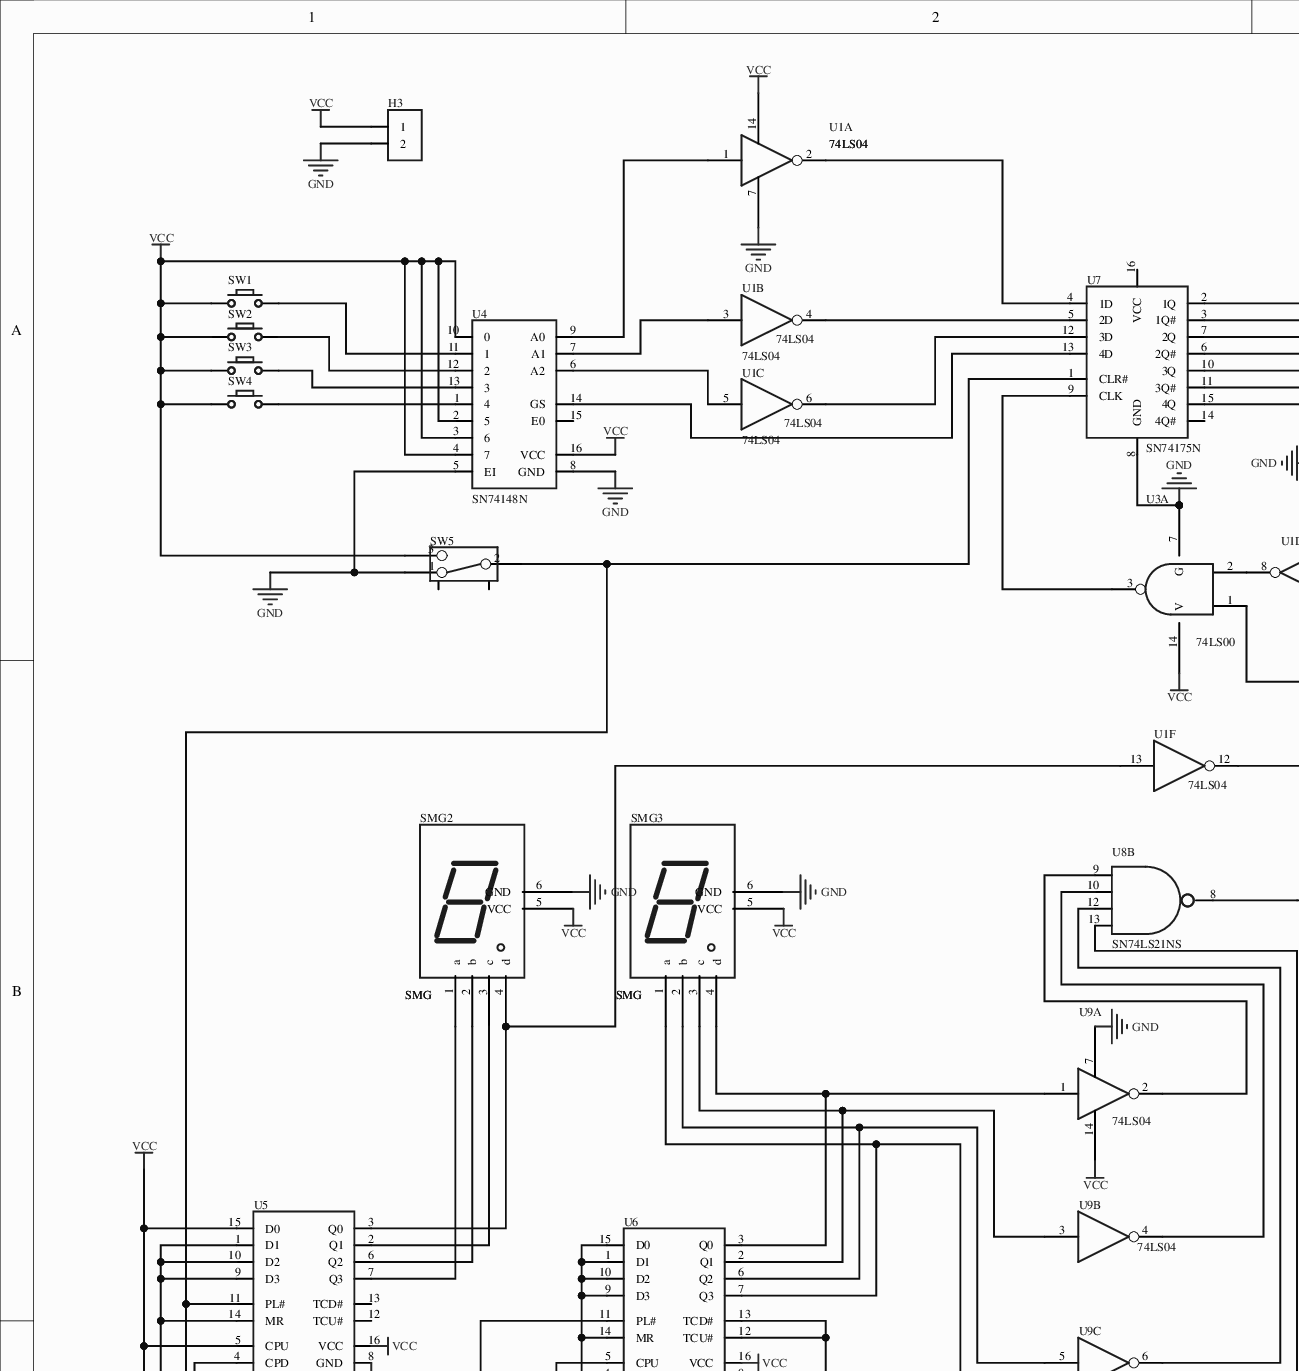
[diagram p0: MISC52149-3.schdoc, top left]
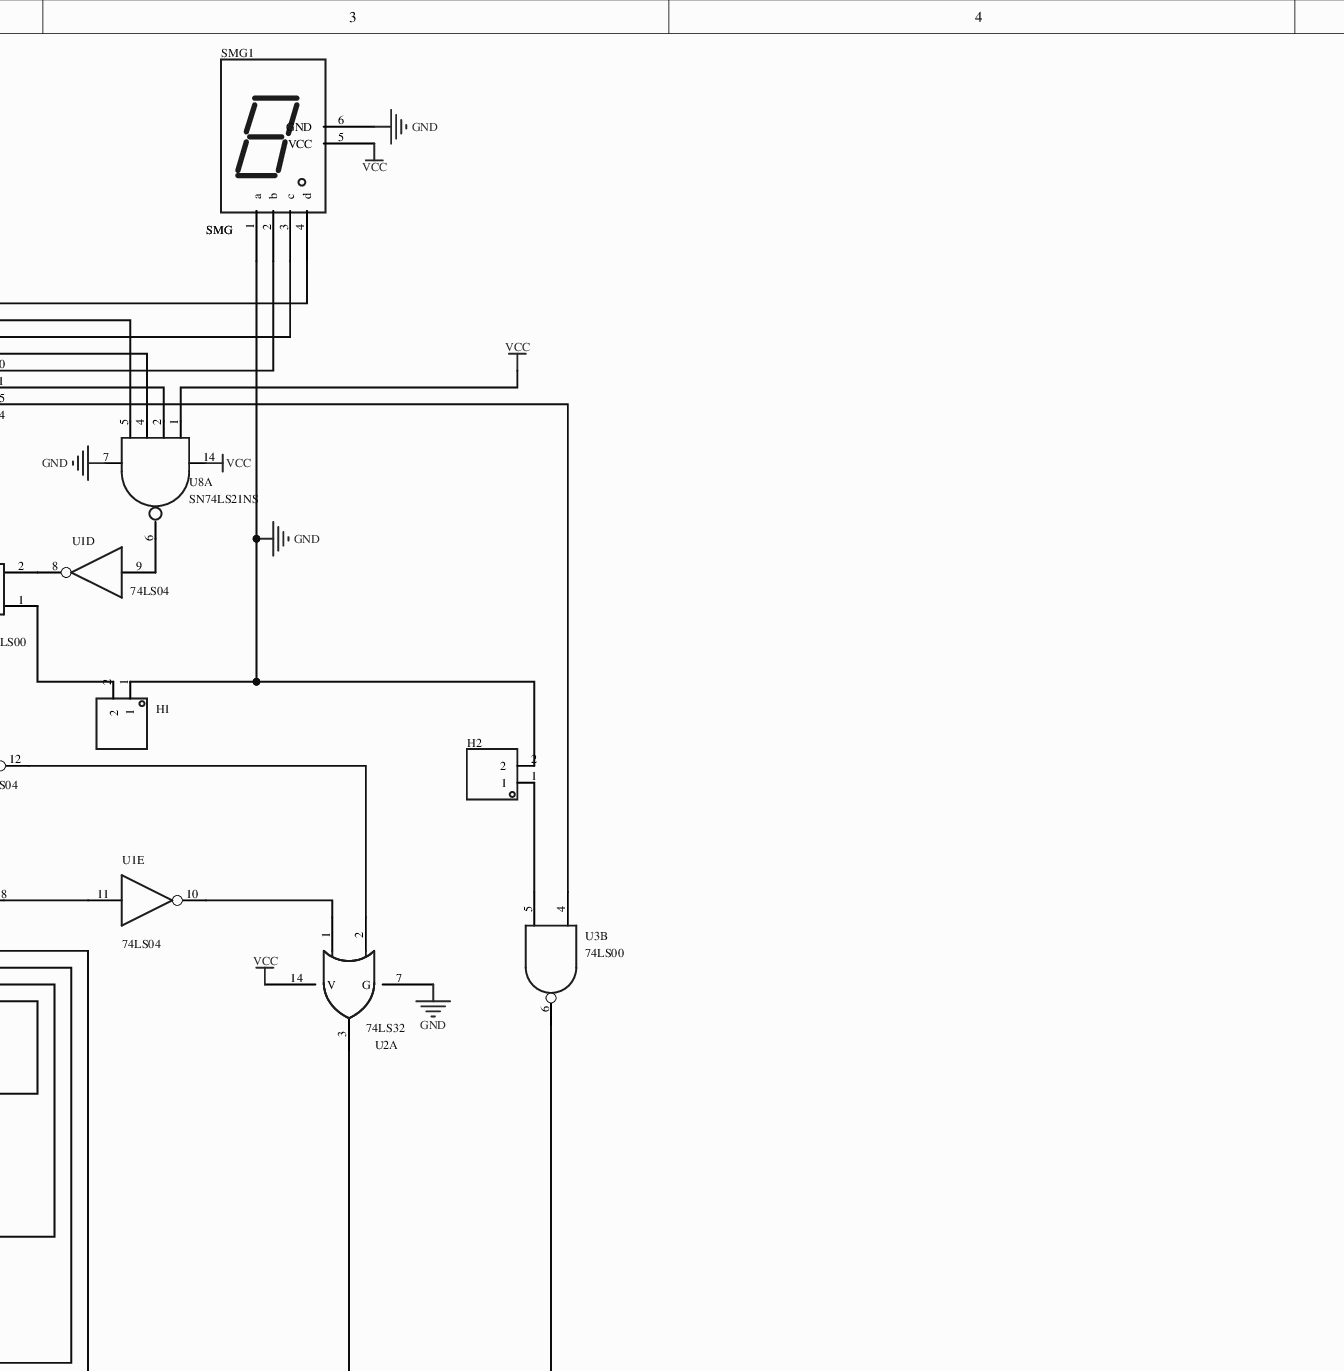
[diagram p1: MISC52149-3.schdoc, top middle]
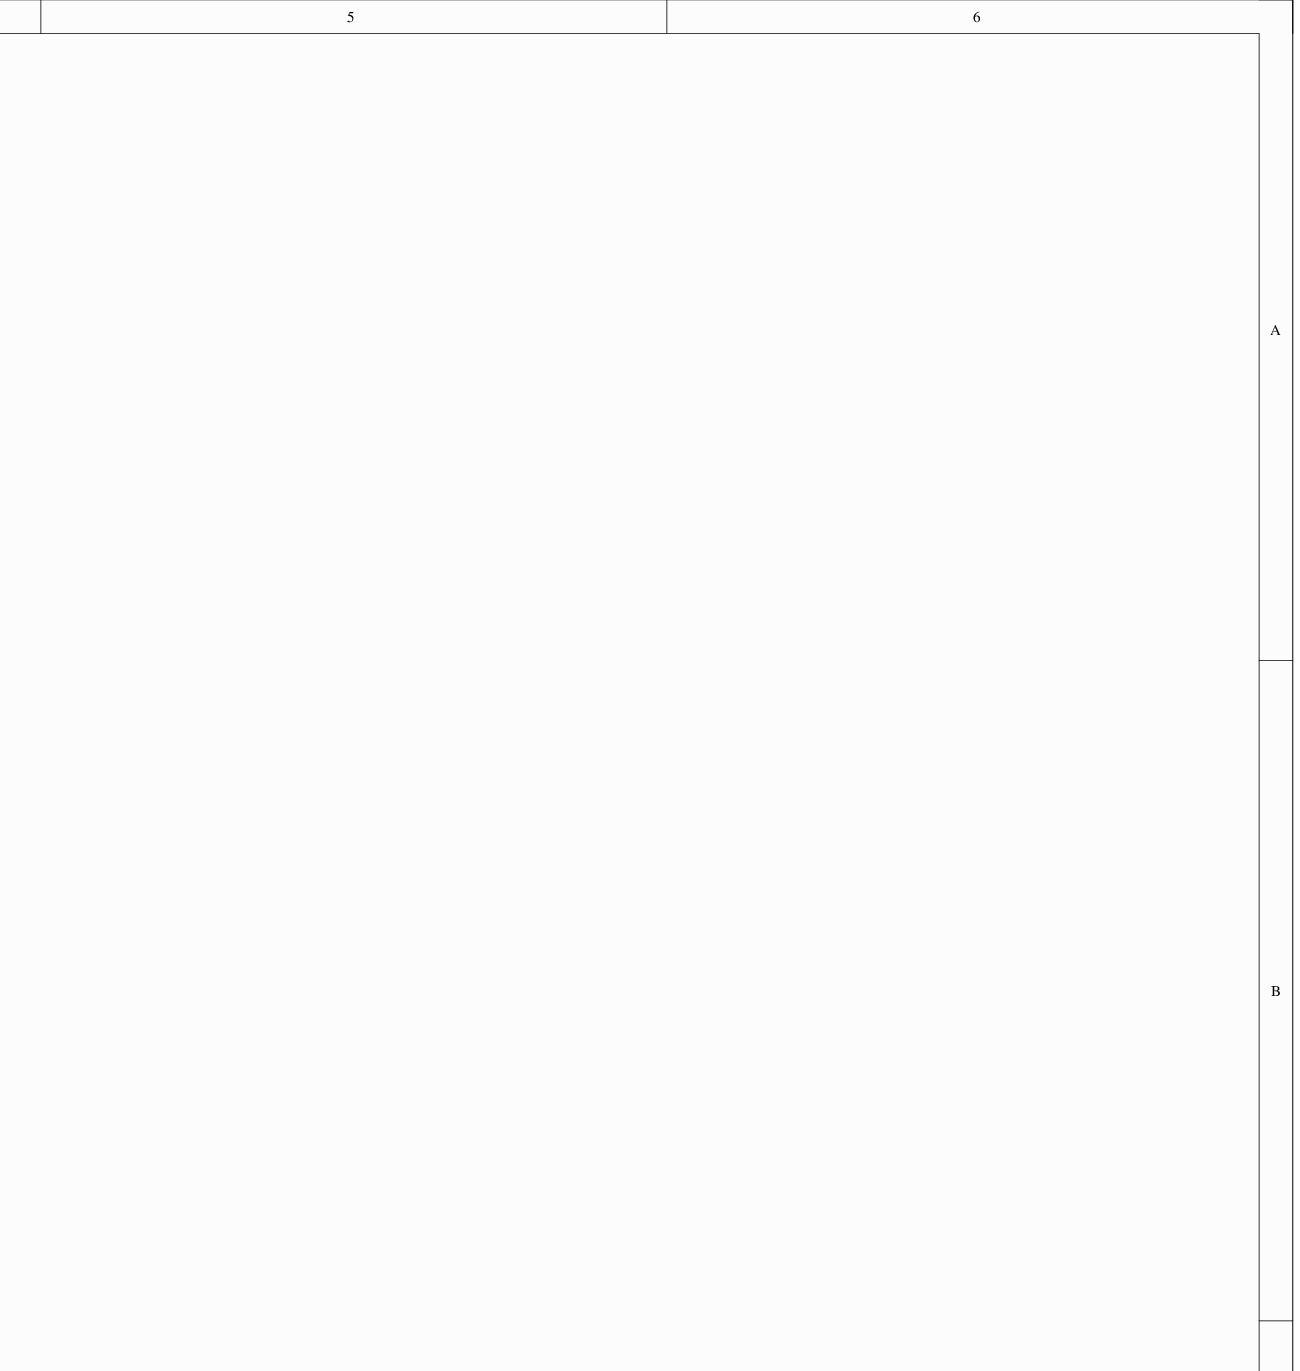
[diagram p2: MISC52149-3.schdoc, top right]
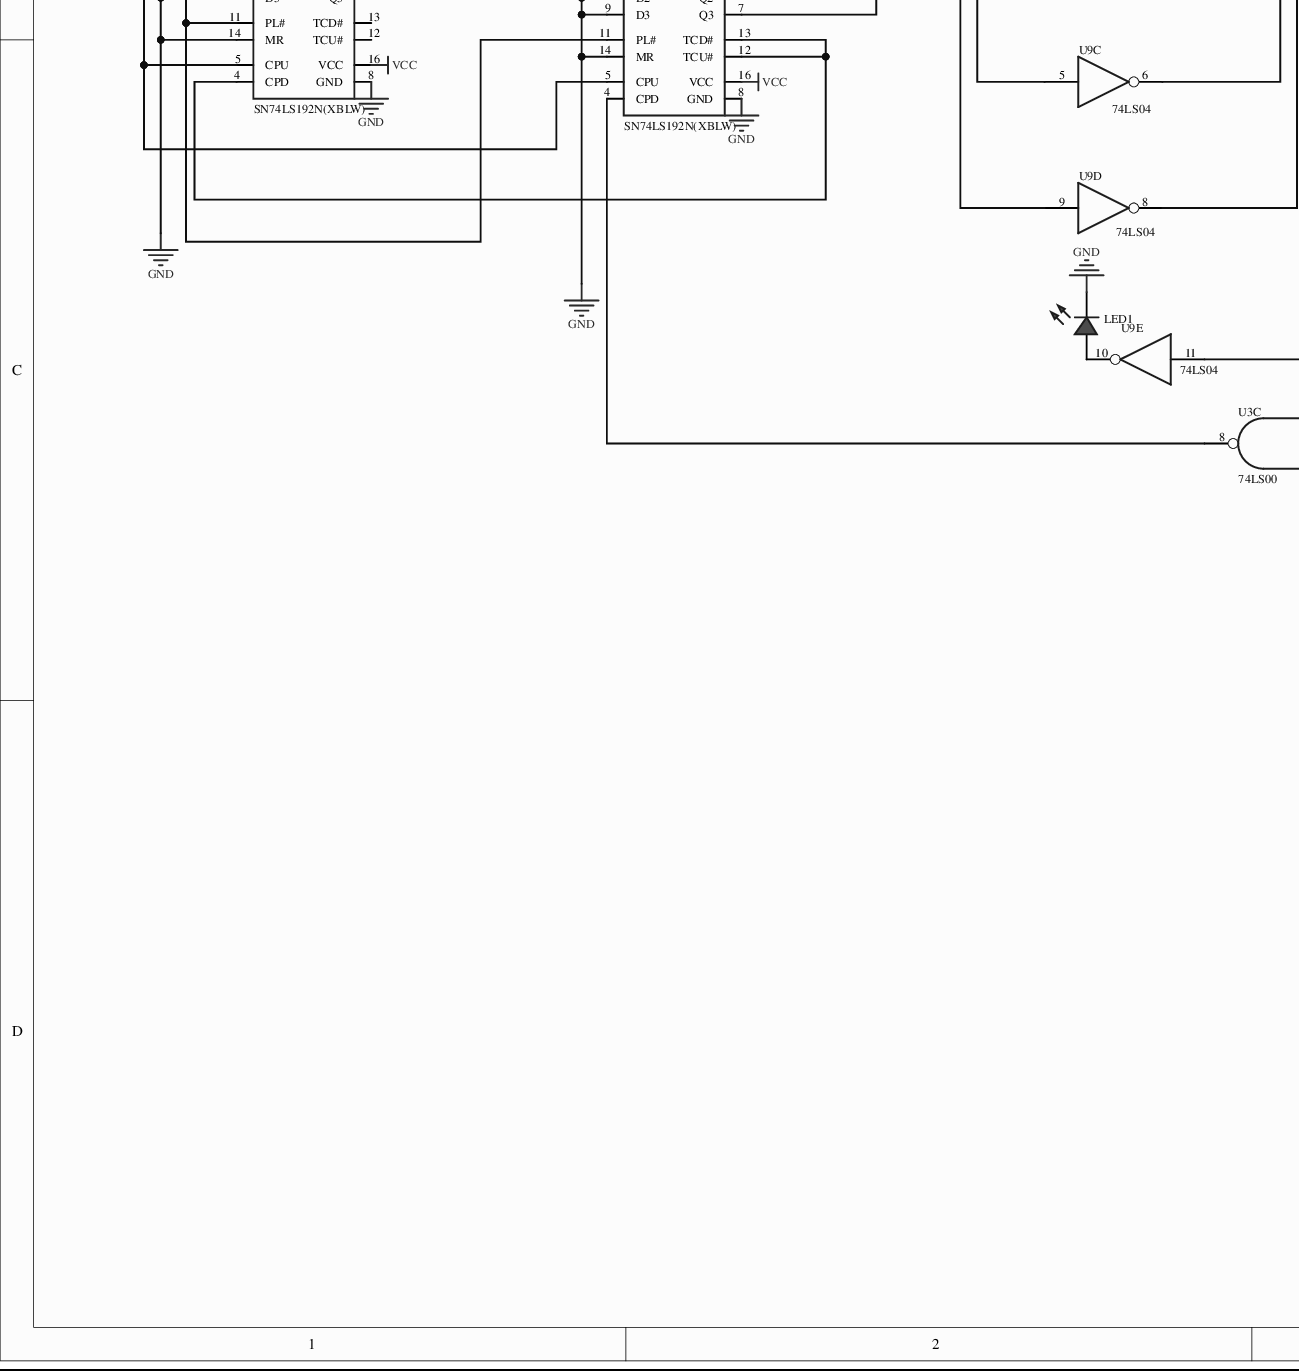
[diagram p3: MISC52149-3.schdoc, bottom left]
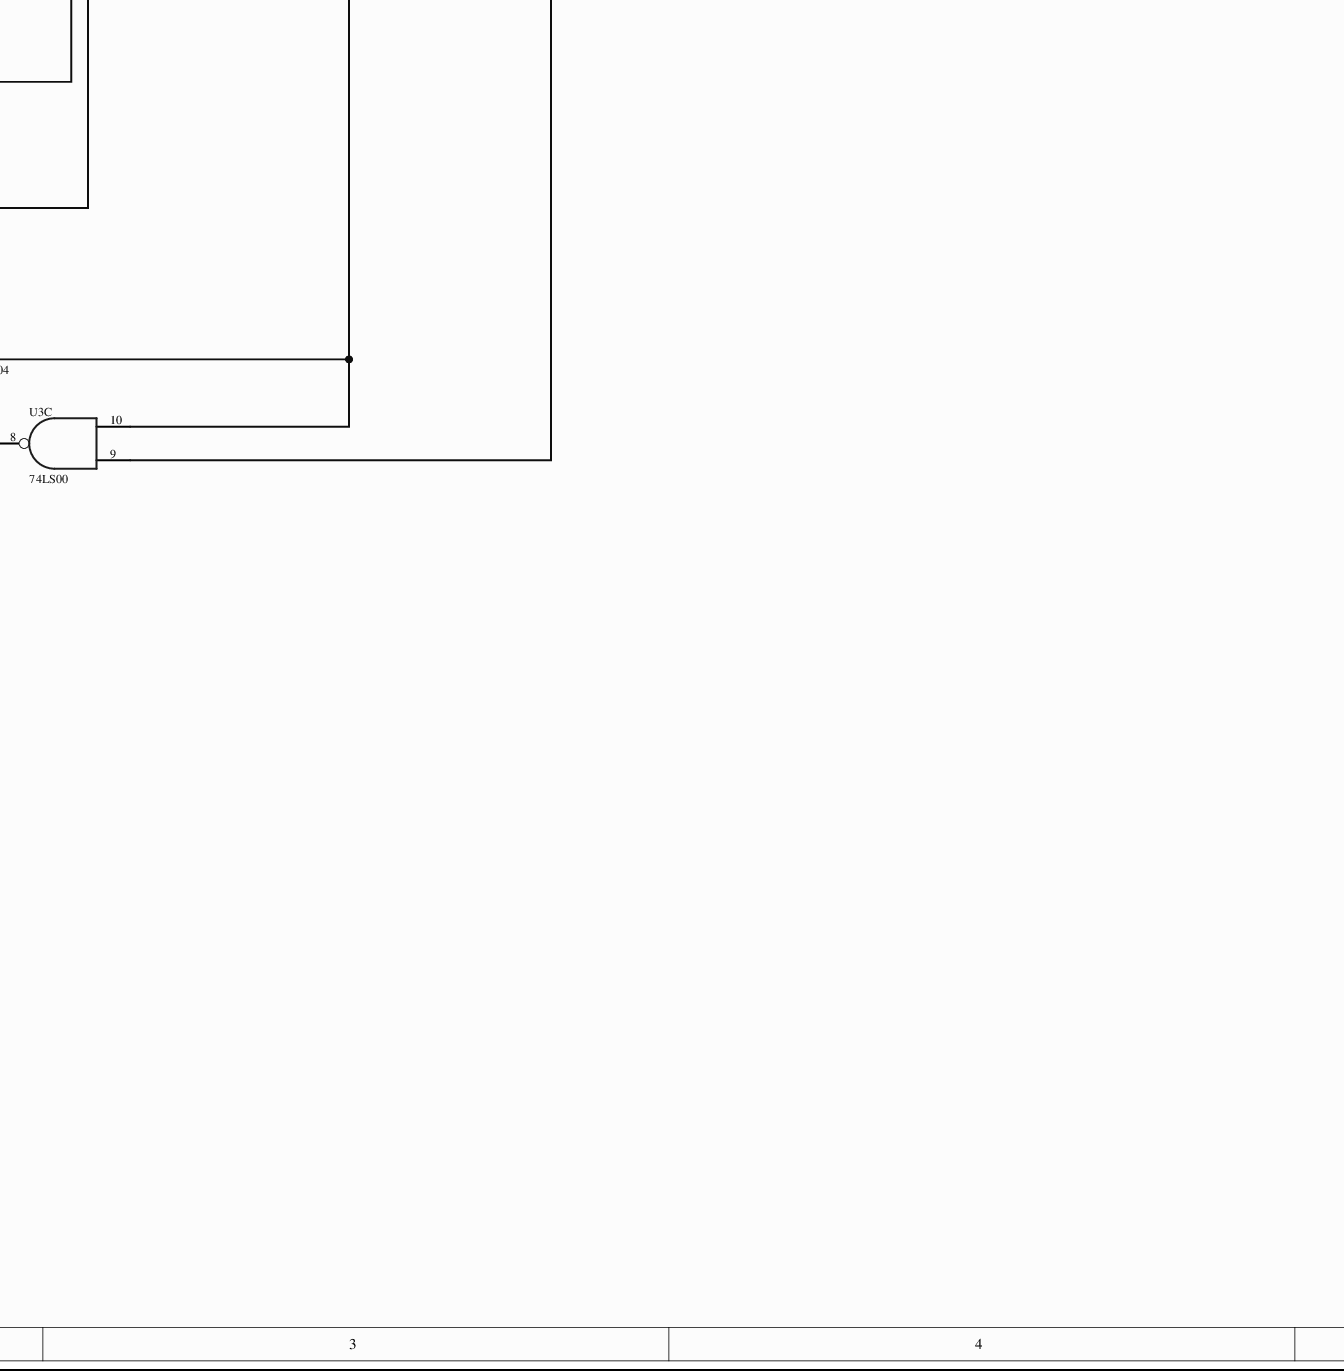
[diagram p4: MISC52149-3.schdoc, bottom middle]
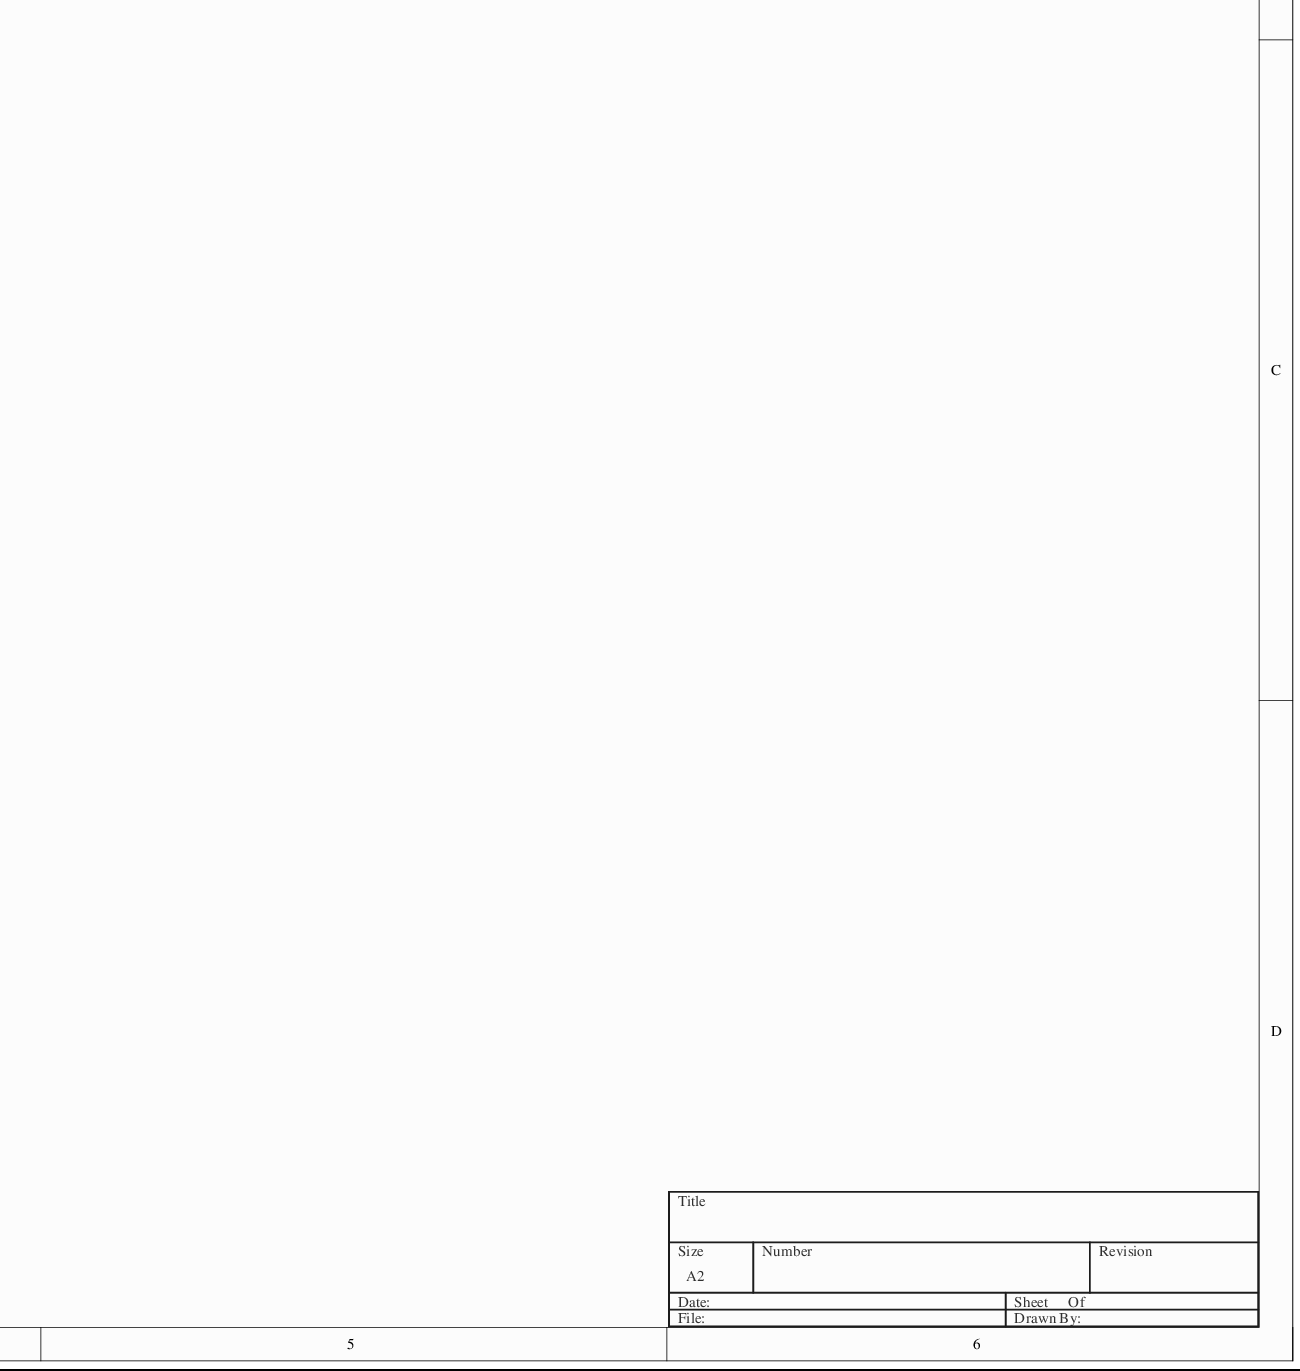
[diagram p5: MISC52149-3.schdoc, bottom right]
# Altium project MISC52149-2.PrjPcb
1 sheet, 21 parts. Net scope: global (net labels, ports and power ports of the same name join across sheets).
Board file: MISC52149.pcbdoc

## Sheet MISC52149-3.schdoc
size 566 x 399 mm

### Parts
H1  (no value)  [HDR-TH_2P-P2.54-V-M-1]
H2  (no value)  [HDR-TH_2P-P2.54-V-M-1]
H3  (no value)  [HDR-TH_2P-P2.54-V-F]
LED1  (no value)  [LED_TH-3mm]
SMG1  SMG  [B含CD译码器的数码管]
SMG2  SMG  [B含CD译码器的数码管]
SMG3  SMG  [B含CD译码器的数码管]
SW1  (no value)  [Key_TH_3.5x6x4.3]
SW2  (no value)  [Key_TH_3.5x6x4.3]
SW3  (no value)  [Key_TH_3.5x6x4.3]
SW4  (no value)  [Key_TH_3.5x6x4.3]
SW5  (no value)  [拨动开关]
U1  74LS04  [DIP-014]  (parts A,B,C,D,E,F of 6)
U2  74LS32  [DIP-014]  (part A of 4)
U3  74LS00  [DIP-014]  (parts A,B,C of 4)
U4  SN74148N  [PDIP-16_L19.3-W6.4-P2.54-LS7.9-BL]
U5  SN74LS192N(XBLW)  [PDIP-16_L19.3-W6.4-P2.54-LS7.94-BL]
U6  SN74LS192N(XBLW)  [PDIP-16_L19.3-W6.4-P2.54-LS7.94-BL]
U7  SN74175N  [DIP-16_L19.3-W6.4-P2.54-LS7.6-BL]
U8  SN74LS21NS  [SOIC-14_L10.0-W5.5-P1.27-LS7.8-BL]  (parts A,B of 2)
U9  74LS04  [DIP-014]  (parts A,B,C,D,E of 6)

### Nets
GND: H1.1 H2.2 H3.2 LED1.2(A) SMG1.1(a) SMG1.6(GND) SMG2.6(GND) SMG3.6(GND) SW5.1 U1.7 U2.7(G) U3.7(G) U4.5(EI) U4.8(GND) U5.1(D1) U5.8(GND) U5.9(D3) U5.10(D2) U5.14(MR) U6.1(D1) U6.8(GND) U6.9(D3) U6.10(D2) U6.14(MR) U6.15(D0) U7.8(GND) U8.7(GND) U9.7
VCC: H3.1 SMG1.5(VCC) SMG2.5(VCC) SMG3.5(VCC) SW1.A SW2.A SW3.A SW4.A SW5.3 U1.14 U2.14(V) U3.14(V) U4.2(5) U4.3(6) U4.4(7) U4.10(0) U4.16(VCC) U5.5(CPU) U5.15(D0) U5.16(VCC) U6.5(CPU) U6.16(VCC) U8.1(1A) U8.14(VCC) U9.14
NetH1_2: H1.2 U3.1(A)
NetH2_1: H2.1 U3.5(B)
NetLED1_1: LED1.1(C) U9.10(Y)
NetSMG1_2: SMG1.2(b) U7.10(3Q)
NetSMG1_3: SMG1.3(c) U7.7(2Q)
NetSMG1_4: SMG1.4(d) U7.2(1Q)
NetSMG2_1: SMG2.1(a) U5.7(Q3)
NetSMG2_2: SMG2.2(b) U5.6(Q2)
NetSMG2_3: SMG2.3(c) U5.2(Q1)
NetSMG2_4: SMG2.4(d) U1.13(A) U5.3(Q0)
NetSMG3_1: SMG3.1(a) U6.7(Q3) U9.9(A)
NetSMG3_2: SMG3.2(b) U6.6(Q2) U9.5(A)
NetSMG3_3: SMG3.3(c) U6.2(Q1) U9.3(A)
NetSMG3_4: SMG3.4(d) U6.3(Q0) U9.1(A)
NetSW1_B: SW1.B U4.11(1)
NetSW2_B: SW2.B U4.12(2)
NetSW3_B: SW3.B U4.13(3)
NetSW4_B: SW4.B U4.1(4)
NetSW5_2: SW5.2 U5.11(PL#) U6.11(PL#) U7.1(CLR#)
NetU1_1: U1.1(A) U4.9(A0)
NetU1_2: U1.2(Y) U7.4(1D)
NetU1_3: U1.3(A) U4.7(A1)
NetU1_4: U1.4(Y) U7.5(2D)
NetU1_5: U1.5(A) U4.6(A2)
NetU1_6: U1.6(Y) U7.12(3D)
NetU1_8: U1.8(Y) U3.2(B)
NetU1_9: U1.9(A) U8.6(1Y)
NetU1_10: U1.10(Y) U2.1(A)
NetU1_11: U1.11(A) U8.8(2Y)
NetU1_12: U1.12(Y) U2.2(B)
NetU2_3: U2.3(Y) U3.10(B) U9.11(A)
NetU3_3: U3.3(Y) U7.9(CLK)
NetU3_4: U3.4(A) U7.15(4Q)
NetU3_6: U3.6(Y) U3.9(A)
NetU3_8: U3.8(Y) U6.4(CPD)
NetU4_14: U4.14(GS) U7.13(4D)
NetU5_4: U5.4(CPD) U6.12(TCU#) U6.13(TCD#)
NetU7_3: U7.3(1Q#) U8.5(1D)
NetU7_6: U7.6(2Q#) U8.4(1C)
NetU7_11: U7.11(3Q#) U8.2(1B)
NetU8_9: U8.9(2A) U9.2(Y)
NetU8_10: U8.10(2B) U9.4(Y)
NetU8_12: U8.12(2C) U9.6(Y)
NetU8_13: U8.13(2D) U9.8(Y)

Not connected (* = marked no-connect by the designer): SW5 4 5; U4 15(E0)*; U5 12(TCU#)* 13(TCD#)*; U7 14(4Q#) 16(VCC)

### Notes on the sheet
- Title
- File:
- Date:
- Size
- A2
- Number
- Drawn By:
- Sheet
- Of
- Revision

### Library data of the parts
H1 H2 = HDR-M_2.54_1x2P: Symbol: 210S-1*2P L=11.6MMGold-plated black; ConvertToPcb: yes; ModelId: 79b2e9f2d70a4d68a1b7098f27c6d4c50819f05c4eef4c71ace90d822a990e87; ModelName: HDR-M-2.54_1x2; ModelTransform: 200,100,0,0,0,0,0,0,-118.11; Device: HDR-M_2.54_1x2P; AddInBom: yes; SupplierPart: C124375; Supplier Footprint: 插件; FootprintName: HDR-TH_2P-P2.54-V-M-1
H3 = HDR-F_2.54_1x2P: Symbol: Header-Female-2.54_1x2; ConvertToPcb: yes; ModelId: a9450ef445564560a104363b9aacde4e0819f05c4eef4c71ace90d822a990e87; ModelName: HDR-TH_2P-P2.54-F-LI-1X2P; ModelTransform: 215.7476,98.425,0,0,0,0,0,0,-129.921; Device: HDR-F_2.54_1x2P; AddInBom: yes; SupplierPart: C49661; Supplier Footprint: 插件; FootprintName: HDR-TH_2P-P2.54-V-F
LED1 = LED_TH-R_3mm: ConvertToPcb: yes; ModelId: a497c992633541038a38947cdc58012f0819f05c4eef4c71ace90d822a990e87; ModelName: LED-TH-3mm_R; ModelTransform: 141.274,153.327,0,0,0,0,-5.984,0,-137.795; Symbol: LED_TH-R; Device: LED_TH-R_3mm; AddInBom: yes; FootprintName: LED_TH-3mm; Supplier Footprint: 插件
SMG1-SMG3 = SMG: Origin Footprint: BCD-decoder display; AddInBom: yes; Symbol: SMG; Device: SMG; Design Item ID: SMG; Library Name: 1-digit display with decoder; FootprintName: BCD-decoder display; ConvertToPcb: yes
SW1-SW4 = Key_TH_3.5x6x4.3: ConvertToPcb: yes; ModelId: c3523f9014d949d7ba5445190a3178990819f05c4eef4c71ace90d822a990e87; ModelName: SW-TH_L6.0-W3.5-H5.0-P6.5; ModelTransform: 308.49,137.8,335.08,0,0,0,0,0,-129.92; Symbol: Key_TH_3.5x6x4.3; Device: Key_TH_3.5x6x4.3; AddInBom: yes; Supplier Footprint: 插件; FootprintName: Key_TH_3.5x6x4.3
SW5 = 拨动开关_正: Symbol: Toggle switch; Device: Toggle switch_positive; ConvertToPcb: yes; ModelId: 4321fe59a4074cbfb4989553f297c68f0819f05c4eef4c71ace90d822a990e87; ModelName: SW-TH_SS-12D02-VG4; ModelTransform: 370.09,208.7,472.35,0,0,0,0,0,-110; AddInBom: yes; Supplier Footprint: 插件; FootprintName: Toggle switch
U1 U9 = 74LS04: Relevance: []; AddInBom: yes; Symbol: 74LS04; Device: 74LS04; Origin Footprint: DIP-014; Design Item ID: 74LS04; Library Name: 74LS04; FootprintName: DIP-014; ConvertToPcb: yes
U2 = 74LS32: Relevance: []; AddInBom: yes; Symbol: 74LS32; Device: 74LS32; Origin Footprint: DIP-014; Design Item ID: 74LS32; Library Name: 74LS32; FootprintName: DIP-014; ConvertToPcb: yes
U3 = 74LS00: Relevance: []; AddInBom: yes; Symbol: 74LS00; Device: 74LS00; Origin Footprint: DIP-014; Design Item ID: 74LS00; Library Name: 74LS00; FootprintName: DIP-014; ConvertToPcb: yes
U4 = SN74148N: Manufacturer: TI(德州仪器); AddInBom: yes; ModelId: 7f4af0d2434d4264b3d074b3c8a801b50819f05c4eef4c71ace90d822a990e87; ModelTransform: 759.841,311.023,0,0,0,0,0,-0.001,-129.921; Symbol: SN74148N; Device: SN74148N; LCSC Part Name: SN74148N; SupplierPart: C3208880; ManufacturerPart: SN74148N; Supplier Footprint: -; JLCPCB Part Class: Extended Part; Datasheet: https://item.szlcsc.com/datasheet/SN74148N/3771896.html; Supplier: LCSC; ConvertToPcb: yes; FootprintName: PDIP-16_L19.3-W6.4-P2.54-LS7.9-BL; ModelName: PDIP-16_L19.3-W6.4-P2.54-LS7.9-BL
U5 U6 = SN74LS192N(XBLW): Operating voltage:2V~6V; Element count:1; Trigger edge:rising edge; Count rate:40MHz;; Manufacturer: XBLW(芯伯乐); AddInBom: yes; ModelId: 96ff5d01b3074dd183bcbc4cd00a63de0819f05c4eef4c71ace90d822a990e87; ModelTransform: 759.841,322.44,0,0,0,0,0,0,-137.795; Direction: Up counter; down counter; Voltage - Supply: 2V~6V; Number of Elements: 1; Reset: Asynchronous; Timing: Synchronous; Count Rate: 40MHz; Propagation Delay: 19ns; Symbol: SN74LS192N(XBLW); Device: SN74LS192N(XBLW); LCSC Part Name: SN74LS192是一款同步BCD上/下计数器。拥有独立的上/下时钟; SupplierPart: C42451384; ManufacturerPart: SN74LS192N(XBLW); Supplier Footprint: DIP-16; JLCPCB Part Class: Extended Part; Datasheet: https://item.szlcsc.com/datasheet/SN74LS192N(XBLW)/44513582.html; Supplier: LCSC; ConvertToPcb: yes; FootprintName: PDIP-16_L19.3-W6.4-P2.54-LS7.94-BL; ModelName: PDIP-16_L19.3-W6.4-P2.54-LS7.94-BL; Logic Type: -; Trigger Type: Rising edge; Operating Temperature: -20℃~+85℃; Number of Bits per Element: -; Power Dissipation: -
U7 = SN74175N: Manufacturer: TI(德州仪器); Symbol: SN74175N_1; AddInBom: yes; ModelId: 6a0b9f170db542aa9e288f652469859c0819f05c4eef4c71ace90d822a990e87; ModelTransform: 759.841,309.842,0,0,0,0,0,0,-118.11; Device: SN74175N; LCSC Part Name: SN74175N; SupplierPart: C3827593; ManufacturerPart: SN74175N; Supplier Footprint: -; JLCPCB Part Class: Extended Part; Datasheet: https://item.szlcsc.com/datasheet/SN74175N/4396067.html; Supplier: LCSC; ConvertToPcb: yes; FootprintName: DIP-16_L19.3-W6.4-P2.54-LS7.6-BL; ModelName: DIP-16_L19.3-W6.4-P2.54-LS7.6-BL
U8 = SN74LS21NS: Logic type:AND gate; Channels:2; Supply voltage:4.75V~5.25V; Max propagation delay:20ns@5V,15pF;; Manufacturer: TI(德州仪器); Add into BOM: yes; 3D Model: d71596ea19114621a3233067db9e387b0819f05c4eef4c71ace90d822a990e87; 3D Model Transform: 400.379,307.087,0,0,0,0,0.0005,-0.0005,0; Number of Channels: 2; Sink Current: 8mA; Source Current: 400uA; High Level Range (VIH): 3.4V; Low Level Range (VIL): 400mV~500mV; ModelName: SOIC-14_L10.3-W5.3-H2.0-LS7.8-P1.27; Symbol: SN74LS21NS; Device: SN74LS21NS; Convert to PCB: yes; LCSC Part Name: SN74LS21NS; Supplier Part: C4468709; Manufacturer Part: SN74LS21NS; Supplier Footprint: SO-14; JLCPCB Part Class: Extended Part; Supplier: LCSC; Logic Gate Type: AND gate; Supply Voltage: 4.75V~5.25V; Series: 74LS series; Propagation Delay Time: 20ns@5V,15pF; Operating Temperature: 0℃~+70℃; FootprintName: SOIC-14_L10.0-W5.5-P1.27-LS7.8-BL